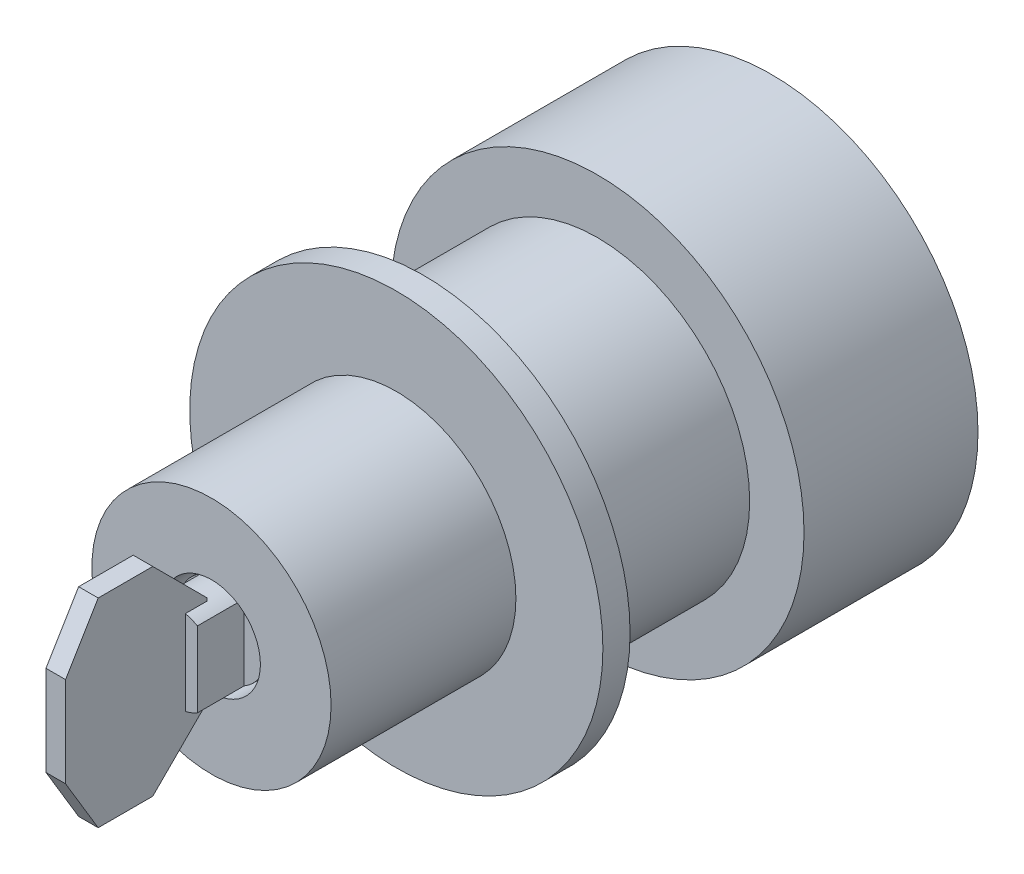
from build123d import *
from OCP.BRepFilletAPI import BRepFilletAPI_MakeChamfer

# Parameters (mm, degrees)
SKETCH_1_R          = 19
EXTRUDE_1_DEPTH     = 16
SKETCH_3_R          = 14
EXTRUDE_2_DEPTH     = 16
SKETCH_4_R          = 19
EXTRUDE_3_DEPTH     = 2.5
SKETCH_5_R          = 11
EXTRUDE_4_DEPTH     = 17
HOLE_WIZARD_1_D     = 9
HOLE_WIZARD_1_DEPTH = 5
SKETCH_7_R          = 4
EXTRUDE_5_DEPTH     = 4
EXTRUDE_6_DEPTH     = 4.3
CUT_EXTRUDE_START   = -2
CUT_EXTRUDE_1_DEPTH = 2
SKETCH_11_W         = 1.8
SKETCH_11_H         = 18.3
EXTRUDE_7_DEPTH     = 13.02
CHAMFER_1_SIZE      = 3
CHAMFER_1_SIZE2     = 5
CHAMFER_2_SIZE      = 5


with BuildPart() as part:
    # 草图1 → 拉伸1 (new body)
    with BuildSketch(Plane.XY):
        Circle(SKETCH_1_R)
    extrude(amount=EXTRUDE_1_DEPTH)

    # 草图3 → 拉伸2 (add)
    with BuildSketch(Plane.XY.offset(16)):
        Circle(SKETCH_3_R)
    extrude(amount=EXTRUDE_2_DEPTH)

    # 草图4 → 拉伸3 (add)
    with BuildSketch(Plane.XY.offset(32)):
        Circle(SKETCH_4_R)
    extrude(amount=EXTRUDE_3_DEPTH)

    # 草图5 → 拉伸4 (add)
    with BuildSketch(Plane.XY.offset(34.5)):
        Circle(SKETCH_5_R)
    extrude(amount=EXTRUDE_4_DEPTH)

    # 孔1
    with Locations(Plane.XY.offset(51.5)):
        with Locations((0, 0)):
            Hole(HOLE_WIZARD_1_D / 2, depth=HOLE_WIZARD_1_DEPTH)

    # 草图7 → 拉伸5 (add)
    with BuildSketch(Plane.XY.offset(46.5)):
        with Locations(Location((0, 0, 0), (0, 0, 180))):
            Circle(SKETCH_7_R)
    extrude(amount=EXTRUDE_5_DEPTH)

    # 草图9 → 拉伸6 (add)
    with BuildSketch(Plane.XY.offset(50.5)):
        with BuildLine():
            Line((-2, 3.464101615), (-2, -3.464101615))
            ThreePointArc((-2, -3.464101615), (0, -4), (2, -3.464101615))
            Line((2, -3.464101615), (2, 3.464101615))
            ThreePointArc((2, 3.464101615), (0, 4), (-2, 3.464101615))
        make_face()
    extrude(amount=EXTRUDE_6_DEPTH)

    # 草图10 → 切除-拉伸1 (cut)
    with BuildSketch(Plane.XY.offset(54.8).offset(CUT_EXTRUDE_START)):
        with BuildLine():
            Line((-0.9, 3.897435054), (-0.9, -3.897435054))
            ThreePointArc((-0.9, -3.897435054), (0, -4), (0.9, -3.897435054))
            Line((0.9, -3.897435054), (0.9, 3.897435054))
            ThreePointArc((0.9, 3.897435054), (0, 4), (-0.9, 3.897435054))
        make_face()
    extrude(amount=CUT_EXTRUDE_1_DEPTH, mode=Mode.SUBTRACT)

    # 草图11 → 拉伸7 (add)
    with BuildSketch(Plane.XY.offset(52.8)):
        Rectangle(SKETCH_11_W, SKETCH_11_H)
    extrude(amount=EXTRUDE_7_DEPTH)

    # 倒角1: one chamfer whose edges measure the first distance from different faces: ONE call of the kernel's chamfer builder (chamfer() names one face for all edges)
    chamfer_1_edges_1 = [part.edges().sort_by_distance(p)[0] for p in [
        (0, 9.15, 65.82),
    ]]
    chamfer_1_side_1 = [part.faces().sort_by_distance(p)[0] for p in [
        (0, 9.15, 59.31),
    ]]
    chamfer_1_edges_2 = [part.edges().sort_by_distance(p)[0] for p in [
        (0, -9.15, 65.82),
    ]]
    chamfer_1_side_2 = [part.faces().sort_by_distance(p)[0] for p in [
        (0, -9.15, 59.31),
    ]]
    chamfer_1 = BRepFilletAPI_MakeChamfer(part.part.solid().wrapped)
    for e in chamfer_1_edges_1:
        chamfer_1.Add(CHAMFER_1_SIZE, CHAMFER_1_SIZE2, e.wrapped, chamfer_1_side_1[0].wrapped)  # the first distance lies on this face
    for e in chamfer_1_edges_2:
        chamfer_1.Add(CHAMFER_1_SIZE, CHAMFER_1_SIZE2, e.wrapped, chamfer_1_side_2[0].wrapped)  # the first distance lies on this face
    add(Compound.cast(chamfer_1.Shape()), mode=Mode.REPLACE)

    # 倒角2
    chamfer_2_edges = [part.edges().sort_by_distance(p)[0] for p in [
        (0, 9.15, 52.8),
        (0, -9.15, 52.8),
    ]]
    chamfer(chamfer_2_edges, length=CHAMFER_2_SIZE)


solid = part.part
